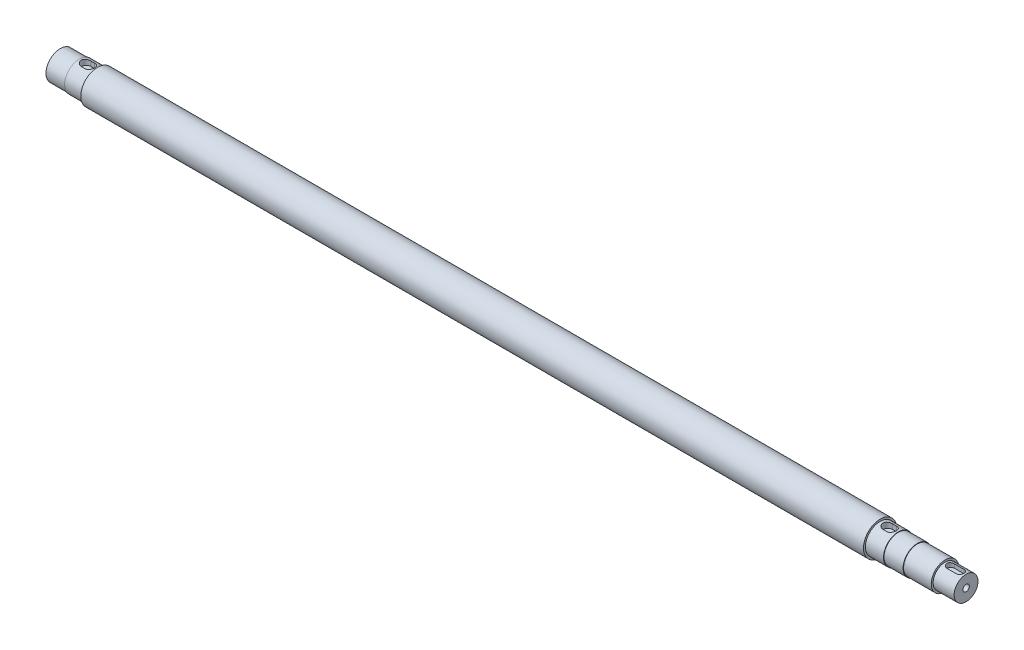
SolidWorks part; units mm, degrees
ref_plane "前视基准面" through (0, 0, 0) normal (0, 0, 1) x (1, 0, 0)
ref_plane "上视基准面" through (0, 0, 0) normal (0, 1, 0) x (1, 0, 0)
ref_plane "右视基准面" through (0, 0, 0) normal (1, 0, 0) x (0, 0, -1)
sketch "草图1" plane through (0, 0, 0) normal (1, 0, 0) x (0, 0, -1)
  circle A0 centre (0, 0) radius 17.5
extrude "凸台-拉伸1" add sketch "草图1" along normal mid plane 820
sketch "草图2" plane through (410, 0, 0) normal (1, 0, 0) x (0, 0, -1)
  circle A0 centre (0, 0) radius 15.5
extrude "凸台-拉伸2" add sketch "草图2" along normal blind 19
sketch "草图3" plane through (429, 0, 0) normal (1, 0, 0) x (0, 0, -1)
  circle A0 centre (0, 0) radius 15
extrude "凸台-拉伸3" add sketch "草图3" along normal blind 20
sketch "草图4" plane through (449, 0, 0) normal (1, 0, 0) x (0, 0, -1)
  circle A0 centre (0, 0) radius 14.5
extrude "凸台-拉伸4" add sketch "草图4" along normal blind 29
sketch "草图5" plane through (478, 0, 0) normal (1, 0, 0) x (0, 0, -1)
  circle A0 centre (0, 0) radius 12.5
extrude "凸台-拉伸5" add sketch "草图5" along normal blind 22
mirror "镜向1" about plane through (0, 0, 0) normal (1, 0, 0) of "凸台-拉伸3", "凸台-拉伸2"
ref_plane "基准面1" through (0, 15.5, 0) normal (0, 1, 0) x (1, 0, 0)
sketch "草图6" plane through (0, 15.5, 0) normal (0, 1, 0) x (1, 0, 0)
  line L0 (-418, 0) -> (-422, 0) construction
  line L1 (-410, 15.5) -> (-410, -15.5) construction
  line L2 (-418, -5) -> (-422, -5)
  line L3 (-418, 5) -> (-422, 5)
  line L4 (422, 0) -> (418, 0) construction
  line L5 (422, -5) -> (418, -5)
  line L6 (422, 5) -> (418, 5)
  line L7 (410, -17.5) -> (410, 17.5) construction
  arc A0 (-418, -5) -> (-418, 5) centre (-418, 0) ccw
  arc A1 (-422, 5) -> (-422, -5) centre (-422, 0) ccw
  arc A2 (422, -5) -> (422, 5) centre (422, 0) ccw
  arc A3 (418, 5) -> (418, -5) centre (418, 0) ccw
  point P5 (-420, 0)
  point P12 (420, 0)
  dimension "D1" = 4
  dimension "D2" = 5
  dimension "D3" = 8
  dimension "D4" = 8
extrude "切除-拉伸1" cut sketch "草图6" against normal blind 5.83
sketch "草图7" plane through (0, 15.5, 0) normal (0, 1, 0) x (1, 0, 0)
  line L0 (484, 0) -> (494, 0) construction
  line L3 (484, 4) -> (494, 4)
  line L4 (484, -4) -> (494, -4)
  line L7 (478, -14.5) -> (478, 14.5) construction
  arc A0 (484, 4) -> (484, -4) centre (484, 0) ccw
  arc A1 (494, -4) -> (494, 4) centre (494, 0) ccw
  point P2 (489, 0)
  dimension "D1" = 10
  dimension "D3" = 6
  dimension "D2" = 4
extrude "切除-拉伸2" cut sketch "草图7" against normal blind 7.66
hole_wizard "M8 螺纹孔1" positions "草图9" profile "草图8" tap size "M8" standard "Iso"
sketch "草图9" plane through (500, 0, 0) normal (1, 0, 0) x (0, 0, -1)
  point P0 (0, 0)
sketch "草图8" plane through (500, 0, 0) normal (0, 1, 0) x (0, 0, -1)
  line L0 (0, 0) -> (0, 22.0429)
  line L1 (0, 22.0429) -> (3.4, 20)
  line L2 (3.4, 20) -> (3.4, 0)
  line L5 (3.4, 0) -> (0, 0)
  line L10 (0, 22.0429) -> (-3.4, 20) construction
  line L11 (0, -6.35) -> (0, 107.95) construction
  dimension "螺纹孔钻头直径" = 6.8
  dimension "螺纹孔钻头深度" = 20
  dimension "导头角度" = 118
cosmetic thread "孔螺蚊线1" parameters "D1"=16, "D2"=8
